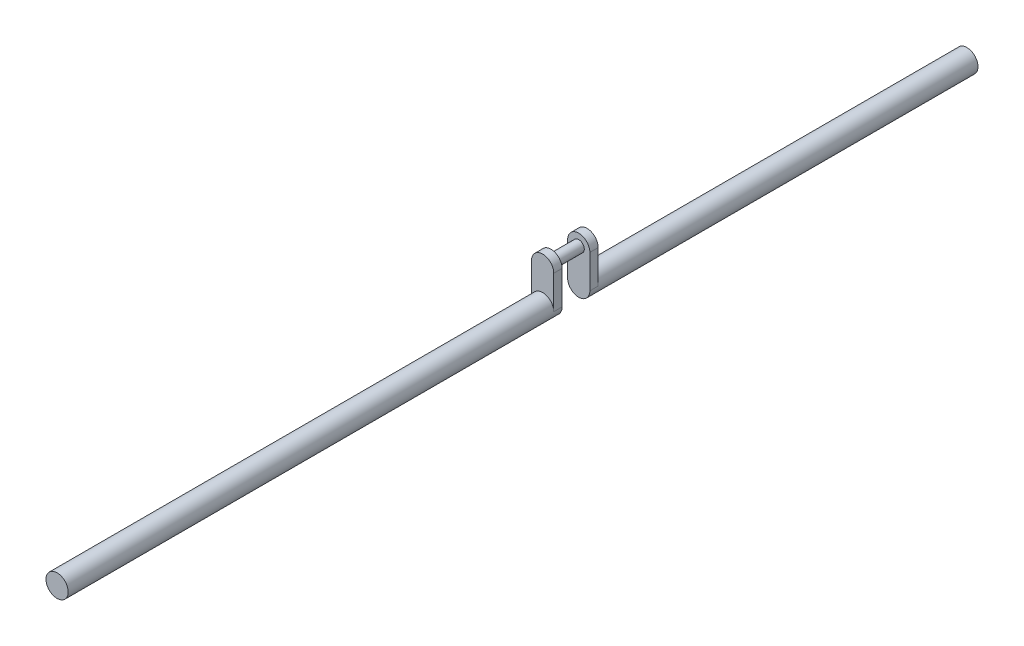
from build123d import *

# Parameters (mm, degrees)
SKETCH1_R               = 10
BOSS_EXTRUDE1_DEPTH     = 362
CUT_EXTRUDE1_DEPTH      = 363.276137773
CUT_EXTRUDE1_DEPTH_BACK = 363.276137773
SKETCH2_W               = 145.080809864
SKETCH2_H               = 40
BOSS_EXTRUDE2_DEPTH     = 20
CUT_EXTRUDE2_DEPTH      = 365.751970522
CUT_EXTRUDE2_DEPTH_BACK = 365.751970522
SKETCH4_W               = 25
SKETCH4_H               = 210.962257982
SKETCH5_R               = 5
BOSS_EXTRUDE3_DEPTH     = 12.5
SKETCH6_R               = 10
BOSS_EXTRUDE4_DEPTH     = 95.2


with BuildPart() as part:
    # Sketch1 → Boss-Extrude1 (new, symmetric)
    with BuildSketch(Plane.XY):
        Circle(SKETCH1_R)
    extrude(amount=BOSS_EXTRUDE1_DEPTH, both=True)

    # Sketch2 → Cut-Extrude1 (cut, two sides: drawn at the far end of the back side and taken through both)
    with BuildSketch(Plane(origin=(0, 0, 0), x_dir=(1, 0, 0), z_dir=(0, 1, 0)).offset(-CUT_EXTRUDE1_DEPTH_BACK)):
        Rectangle(SKETCH2_W, SKETCH2_H)
    extrude(amount=CUT_EXTRUDE1_DEPTH + CUT_EXTRUDE1_DEPTH_BACK, mode=Mode.SUBTRACT)


with BuildPart() as cut_extrude1_piece_1:
    # of the separate pieces the step leaves, piece 1, a body of its own (cut_extrude1_pieces)
    add(part.part.solids().sort_by_distance((10, 0, -362))[0])



with BuildPart() as cut_extrude1_piece_2:
    # of the separate pieces the step leaves, piece 2, a body of its own (cut_extrude1_pieces)
    add(part.part.solids().sort_by_distance((10, 0, 20))[0])


with BuildPart() as cut_extrude1_piece_1_1:
    add(cut_extrude1_piece_1.part)

    add(cut_extrude1_piece_2.part)  # Boss-Extrude2 merges Cut-Extrude1 piece 2
    # Sketch3 → Boss-Extrude2 (add, symmetric)
    with BuildSketch(Plane.XY):
        with BuildLine():
            Line((-10, 0), (-10, 30))
            ThreePointArc((-10, 30), (0, 40), (10, 30))
            Line((10, 30), (10, 0))
            ThreePointArc((10, 0), (0, -10), (-10, 0))
        make_face()
    extrude(amount=BOSS_EXTRUDE2_DEPTH, both=True)

    # Sketch4 → Cut-Extrude2 (cut, two sides: drawn at the far end of the back side and taken through both)
    with BuildSketch(Plane(origin=(10, 0, 0), x_dir=(0, 0, -1), z_dir=(1, 0, 0)).offset(-CUT_EXTRUDE2_DEPTH_BACK)):
        Rectangle(SKETCH4_W, SKETCH4_H)
    extrude(amount=CUT_EXTRUDE2_DEPTH + CUT_EXTRUDE2_DEPTH_BACK, mode=Mode.SUBTRACT)


with BuildPart() as cut_extrude2_piece_1:
    # of the separate pieces the step leaves, piece 1, a body of its own (cut_extrude2_pieces)
    add(cut_extrude1_piece_1_1.part.solids().sort_by_distance((10, 0, 20))[0])



with BuildPart() as cut_extrude2_piece_2:
    # of the separate pieces the step leaves, piece 2, a body of its own (cut_extrude2_pieces)
    add(cut_extrude1_piece_1_1.part.solids().sort_by_distance((10, 0, -20))[0])


with BuildPart() as cut_extrude2_piece_1_1:
    add(cut_extrude2_piece_1.part)

    add(cut_extrude2_piece_2.part)  # Boss-Extrude3 merges Cut-Extrude2 piece 2
    # Sketch5 → Boss-Extrude3 (add, symmetric)
    with BuildSketch(Plane.XY):
        with Locations(Location((0, 30, 0), (0, 0, 180))):
            Circle(SKETCH5_R)
    extrude(amount=BOSS_EXTRUDE3_DEPTH, both=True)

    # Sketch6 → Boss-Extrude4 (add)
    with BuildSketch(Plane.XY.offset(362)):
        Circle(SKETCH6_R)
    extrude(amount=BOSS_EXTRUDE4_DEPTH)


solid = cut_extrude2_piece_1_1.part
